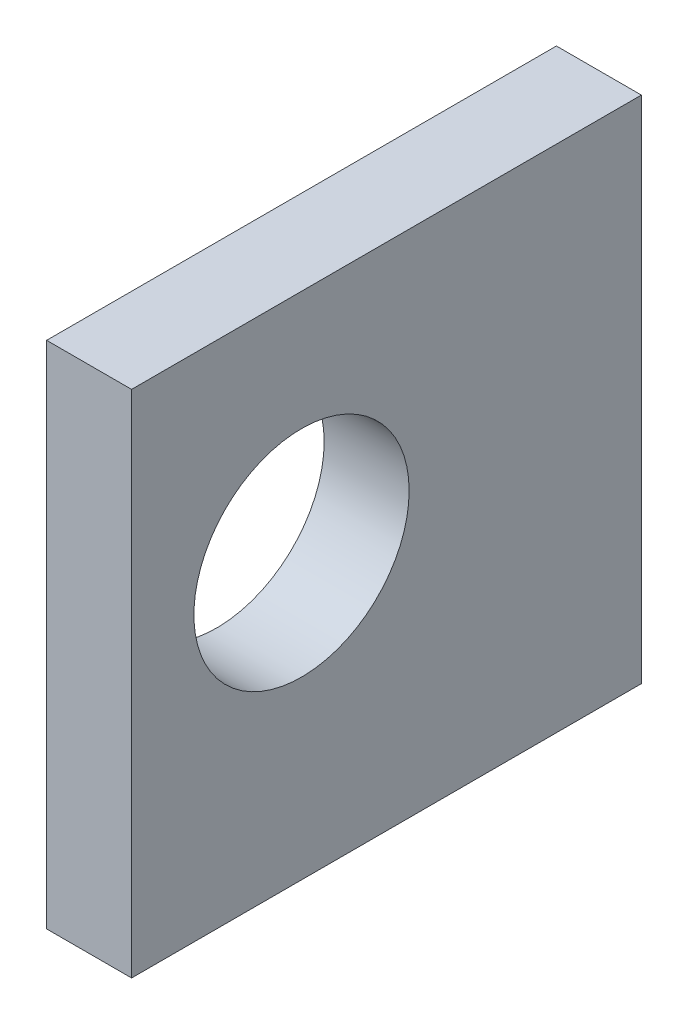
SolidWorks part; units mm, degrees
material "Q235-A"
ref_plane "Front Plane" through (0, 0, 0) normal (0, 0, 1) x (1, 0, 0)
ref_plane "Top Plane" through (0, 0, 0) normal (0, 1, 0) x (1, 0, 0)
ref_plane "Right Plane" through (0, 0, 0) normal (1, 0, 0) x (0, 0, -1)
sketch "Sketch1" plane through (0, 0, 0) normal (1, 0, 0) x (0, 0, -1)
  line L1 (45, -45) -> (-45, -45)
  line L2 (45, -45) -> (45, 45)
  line L3 (45, 45) -> (-45, 45)
  line L4 (-45, -45) -> (-45, 45)
  line L5 (45, -45) -> (-45, 45) construction
  line L6 (45, 45) -> (-45, -45) construction
  point P0 (0, 0)
  dimension "D1" = 90
  dimension "D2" = 90
extrude "Boss-Extrude1" add sketch "Sketch1" along normal mid plane 15
sketch "Sketch2" plane through (7.5, 0, 0) normal (1, 0, 0) x (0, 0, -1)
  line L0 (0, 5) -> (-15, 5) construction
  line L1 (-45, 45) -> (-45, -45) construction
  line L2 (0, 0) -> (-6.6557, 0) construction
  circle A0 centre (-15, 5) radius 19
  dimension "D1" = 38
  dimension "D2" = 30
  dimension "D3" = 5
extrude "Cut-Extrude1" cut sketch "Sketch2" against normal blind 15
